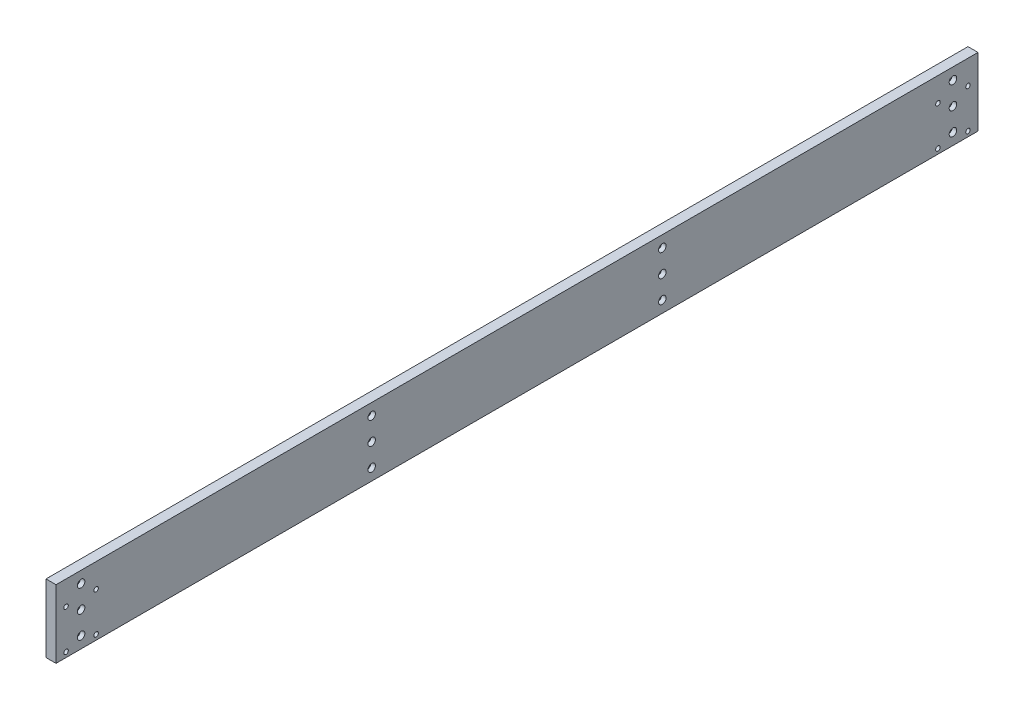
from build123d import *

# Parameters (mm, degrees)
SKETCH_2_W                 = 1840
SKETCH_2_H                 = 136
EXTRUDE_2_DEPTH            = 20
HOLE_WIZARD_2_D            = 9
HOLE_WIZARD_2_CBORE_D      = 15
HOLE_WIZARD_2_CBORE_DEPTH  = 9
PATTERN_LINEAR_1_COUNT     = 4
PATTERN_LINEAR_1_PITCH     = 580
HOLE_WIZARD_2_2_AT_2_COUNT = 2
HOLE_WIZARD_2_2_AT_2_PITCH = 60
HOLE_WIZARD_2_2_AT_3_COUNT = 2
HOLE_WIZARD_2_2_AT_3_PITCH = 78
HOLE_WIZARD_2_2_AT_4_COUNT = 2
HOLE_WIZARD_2_2_AT_4_PITCH = 98.407316801
HOLE_WIZARD_2_2_AT_5_COUNT = 2
HOLE_WIZARD_2_2_AT_5_PITCH = 1740
HOLE_WIZARD_2_2_AT_6_COUNT = 2
HOLE_WIZARD_2_2_AT_6_PITCH = 1800
HOLE_WIZARD_2_2_AT_7_COUNT = 2
HOLE_WIZARD_2_2_AT_7_PITCH = 1741.747398448
HOLE_WIZARD_2_2_AT_8_COUNT = 2
HOLE_WIZARD_2_2_AT_8_PITCH = 1801.689207383


with BuildPart() as part:
    # 草图2 → 凸台-拉伸2 (new body)
    with BuildSketch(Plane(origin=(0, 0, 0), x_dir=(0, 0, -1), z_dir=(1, 0, 0))):
        Rectangle(SKETCH_2_W, SKETCH_2_H)
    extrude(amount=EXTRUDE_2_DEPTH)

    # Hole Wizard 2 (through all)
    with Locations(Plane(origin=(20, 0, 0), x_dir=(0, 0, -1), z_dir=(1, 0, 0))):
        with Locations((-870, 45), (-870, -45), (-870, 0)):
            hole_wizard_2 = CounterBoreHole(HOLE_WIZARD_2_D / 2, HOLE_WIZARD_2_CBORE_D / 2, HOLE_WIZARD_2_CBORE_DEPTH)

    # 阵列(线性)1: Hole Wizard 2 ×4
    with Locations(*[(0, 0, -i * PATTERN_LINEAR_1_PITCH) for i in range(1, PATTERN_LINEAR_1_COUNT)]):
        add(hole_wizard_2, mode=Mode.SUBTRACT)

    # 草图6 → Hole Wizard 2 2 (revolve, cut)
    with BuildSketch(Plane(origin=(0, 20, -900), x_dir=(0, 0, 1), z_dir=(0, 1, 0))):
        Polygon((0, 0), (0, 20), (4.5, 20), (4.5, 9), (7.5, 9), (7.5, 0.025), (7.525, 0), align=None)
    hole_wizard_2_2 = revolve(axis=Axis((-6.35, 20, -900), (1, 0, 0)), mode=Mode.SUBTRACT)

    # Hole Wizard 2 2 at 2: Hole Wizard 2 2 ×2
    with Locations(*[(0, 0, i * HOLE_WIZARD_2_2_AT_2_PITCH) for i in range(1, HOLE_WIZARD_2_2_AT_2_COUNT)]):
        add(hole_wizard_2_2, mode=Mode.SUBTRACT)

    # Hole Wizard 2 2 at 3: Hole Wizard 2 2 ×2
    with Locations(*[(0, -i * HOLE_WIZARD_2_2_AT_3_PITCH, 0) for i in range(1, HOLE_WIZARD_2_2_AT_3_COUNT)]):
        add(hole_wizard_2_2, mode=Mode.SUBTRACT)

    # Hole Wizard 2 2 at 4: Hole Wizard 2 2 ×2
    with Locations(*[Vector(0, -0.7926239891046006, 0.6097107608496917) * (i * HOLE_WIZARD_2_2_AT_4_PITCH) for i in range(1, HOLE_WIZARD_2_2_AT_4_COUNT)]):
        add(hole_wizard_2_2, mode=Mode.SUBTRACT)

    # Hole Wizard 2 2 at 5: Hole Wizard 2 2 ×2
    with Locations(*[(0, 0, i * HOLE_WIZARD_2_2_AT_5_PITCH) for i in range(1, HOLE_WIZARD_2_2_AT_5_COUNT)]):
        add(hole_wizard_2_2, mode=Mode.SUBTRACT)

    # Hole Wizard 2 2 at 6: Hole Wizard 2 2 ×2
    with Locations(*[(0, 0, i * HOLE_WIZARD_2_2_AT_6_PITCH) for i in range(1, HOLE_WIZARD_2_2_AT_6_COUNT)]):
        add(hole_wizard_2_2, mode=Mode.SUBTRACT)

    # Hole Wizard 2 2 at 7: Hole Wizard 2 2 ×2
    with Locations(*[Vector(0, -0.0447826131788728, 0.9989967555287012) * (i * HOLE_WIZARD_2_2_AT_7_PITCH) for i in range(1, HOLE_WIZARD_2_2_AT_7_COUNT)]):
        add(hole_wizard_2_2, mode=Mode.SUBTRACT)

    # Hole Wizard 2 2 at 8: Hole Wizard 2 2 ×2
    with Locations(*[Vector(0, -0.04329270535693645, 0.9990624313139183) * (i * HOLE_WIZARD_2_2_AT_8_PITCH) for i in range(1, HOLE_WIZARD_2_2_AT_8_COUNT)]):
        add(hole_wizard_2_2, mode=Mode.SUBTRACT)


solid = part.part
